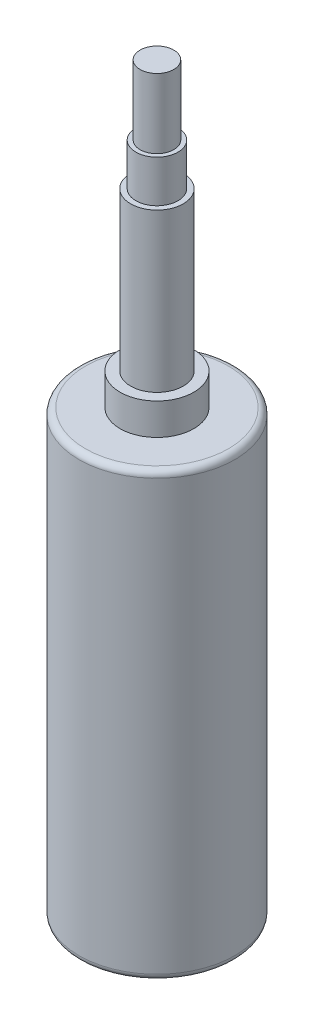
SolidWorks part; units mm, degrees
ref_plane "前视基准面" through (0, 0, 0) normal (0, 0, 1) x (1, 0, 0)
ref_plane "上视基准面" through (0, 0, 0) normal (0, 1, 0) x (1, 0, 0)
ref_plane "右视基准面" through (0, 0, 0) normal (1, 0, 0) x (0, 0, -1)
sketch "草图1" plane through (0, 0, 0) normal (0, 1, 0) x (1, 0, 0)
  circle A0 centre (0, 0) radius 37
  dimension "D1" = 74
extrude "凸台-拉伸1" add sketch "草图1" along normal mid plane 210
sketch "草图2" plane through (0, 105, 0) normal (0, 1, 0) x (1, 0, 0)
  circle A0 centre (0, 0) radius 17.5
  dimension "D1" = 35
extrude "凸台-拉伸2" add sketch "草图2" along normal blind 15
sketch "草图3" plane through (0, 120, 0) normal (0, 1, 0) x (1, 0, 0)
  circle A0 centre (0, 0) radius 12.5
  dimension "D1" = 25
extrude "凸台-拉伸3" add sketch "草图3" along normal blind 75
sketch "草图4" plane through (0, 195, 0) normal (0, 1, 0) x (1, 0, 0)
  circle A0 centre (0, 0) radius 10
  dimension "D1" = 20
extrude "凸台-拉伸4" add sketch "草图4" along normal blind 20
cosmetic thread "装饰螺纹线1" parameters "D1"=14, "D2"=19
sketch "草图5" plane through (0, 215, 0) normal (0, 1, 0) x (1, 0, 0)
  circle A0 centre (0, 0) radius 8
  dimension "D1" = 16
extrude "凸台-拉伸5" add sketch "草图5" along normal blind 33
fillet "圆角1" radius 3 2 edges at (0, -105, 37) (0, 105, 37)
